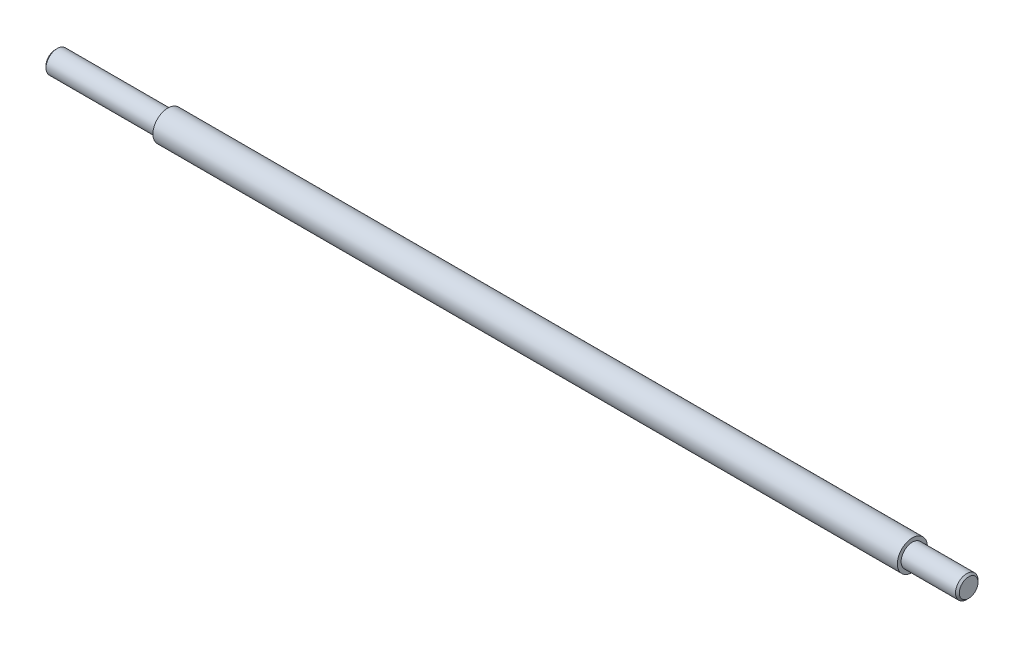
from build123d import *

# Parameters (mm, degrees)
SKETCH1_R           = 8
BOSS_EXTRUDE1_DEPTH = 198.5
SKETCH2_R           = 6
BOSS_EXTRUDE2_DEPTH = 30
BOSS_EXTRUDE3_START = 60
SKETCH3_R           = 6
BOSS_EXTRUDE3_DEPTH = 60
CHAMFER1_SIZE       = 1
CHAMFER2_SIZE       = 1


with BuildPart() as part:
    # Sketch1 → Boss-Extrude1 (new, symmetric)
    with BuildSketch(Plane(origin=(0, 0, 0), x_dir=(0, 0, -1), z_dir=(1, 0, 0))):
        Circle(SKETCH1_R)
    extrude(amount=BOSS_EXTRUDE1_DEPTH, both=True)

    # Sketch2 → Boss-Extrude2 (add)
    with BuildSketch(Plane(origin=(198.5, 0, 0), x_dir=(0, 0, -1), z_dir=(1, 0, 0))):
        Circle(SKETCH2_R)
    extrude(amount=BOSS_EXTRUDE2_DEPTH)

    # Sketch3 → Boss-Extrude3 (add)
    with BuildSketch(Plane.ZY.offset(198.5).offset(BOSS_EXTRUDE3_START)):
        with Locations(Location((0, 0, 0), (0, 0, 180))):
            Circle(SKETCH3_R)
    extrude(amount=-BOSS_EXTRUDE3_DEPTH)

    # Chamfer1
    chamfer1_edges = [part.edges().sort_by_distance(p)[0] for p in [
        (228.5, 0, 6),
    ]]
    chamfer(chamfer1_edges, length=CHAMFER1_SIZE)

    # Chamfer2
    chamfer2_edges = [part.edges().sort_by_distance(p)[0] for p in [
        (-258.5, 0, 6),
    ]]
    chamfer(chamfer2_edges, length=CHAMFER2_SIZE)


solid = part.part
